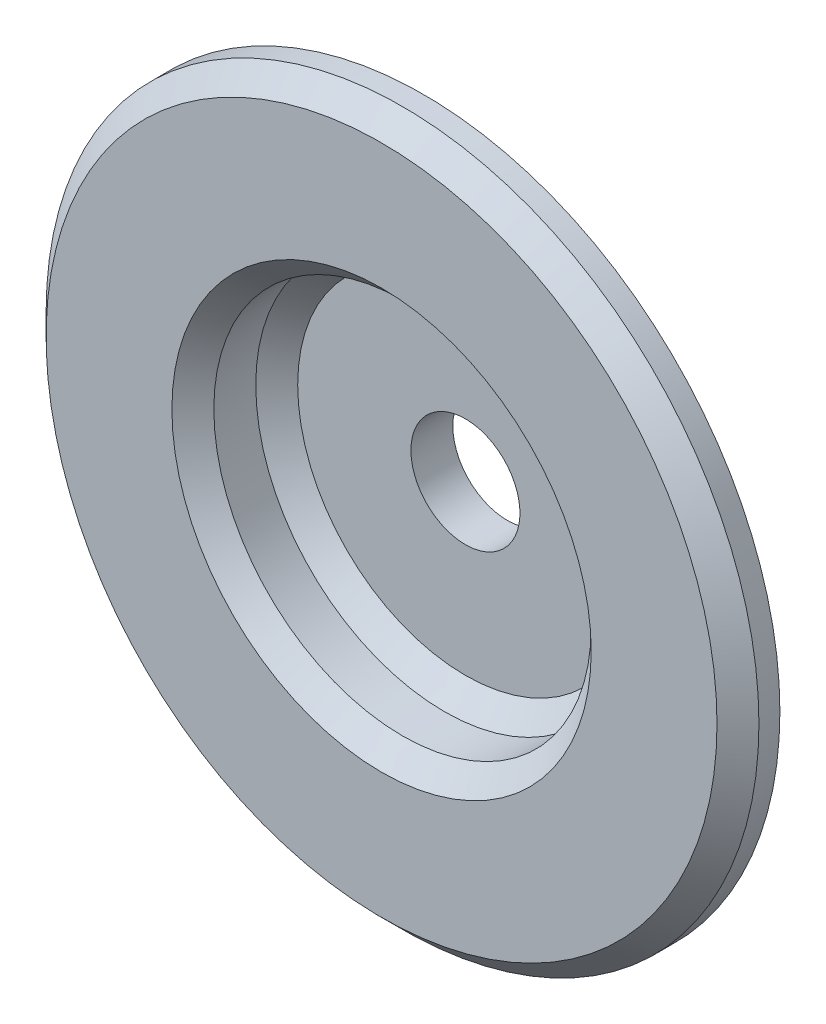
SolidWorks part; units mm, degrees
material "6061 合金"
ref_plane "前视基准面" through (0, 0, 0) normal (0, 0, 1) x (1, 0, 0)
ref_plane "上视基准面" through (0, 0, 0) normal (0, 1, 0) x (1, 0, 0)
ref_plane "右视基准面" through (0, 0, 0) normal (1, 0, 0) x (0, 0, -1)
other "Configuration Table"
sketch "草图1" plane through (0, 0, 0) normal (0, 0, 1) x (1, 0, 0)
  circle A0 centre (0, 0) radius 11
  circle A1 centre (0, 0) radius 9
  dimension "D1" = 22
  dimension "D2" = 2
extrude "凸台-拉伸1" add sketch "草图1" along normal blind 6
sketch "草图2" plane through (0, 0, 0) normal (0, 0, -1) x (-1, 0, 0)
  circle A0 centre (0, 0) radius 2.6
  circle A1 centre (0, 0) radius 11 construction
  circle A2 centre (0, 0) radius 11
  dimension "D1" = 5.2
extrude "凸台-拉伸2" add sketch "草图2" against normal blind 2
chamfer "倒角1" distance 1 angle 45 2 edges at (-9, 0, 2) (11, 0, 0)
sketch "草图3" plane through (0, 0, 6) normal (0, 0, 1) x (1, 0, 0)
  circle A0 centre (0, 0) radius 17
  circle A1 centre (0, 0) radius 11 construction
  circle A2 centre (0, 0) radius 9 construction
  circle A3 centre (0, 0) radius 9
  dimension "D1" = 6
extrude "凸台-拉伸3" add sketch "草图3" against normal blind 2
chamfer "倒角2" distance 1 angle 45 2 edges at (17, 0, 6) (9, 0, 6)
